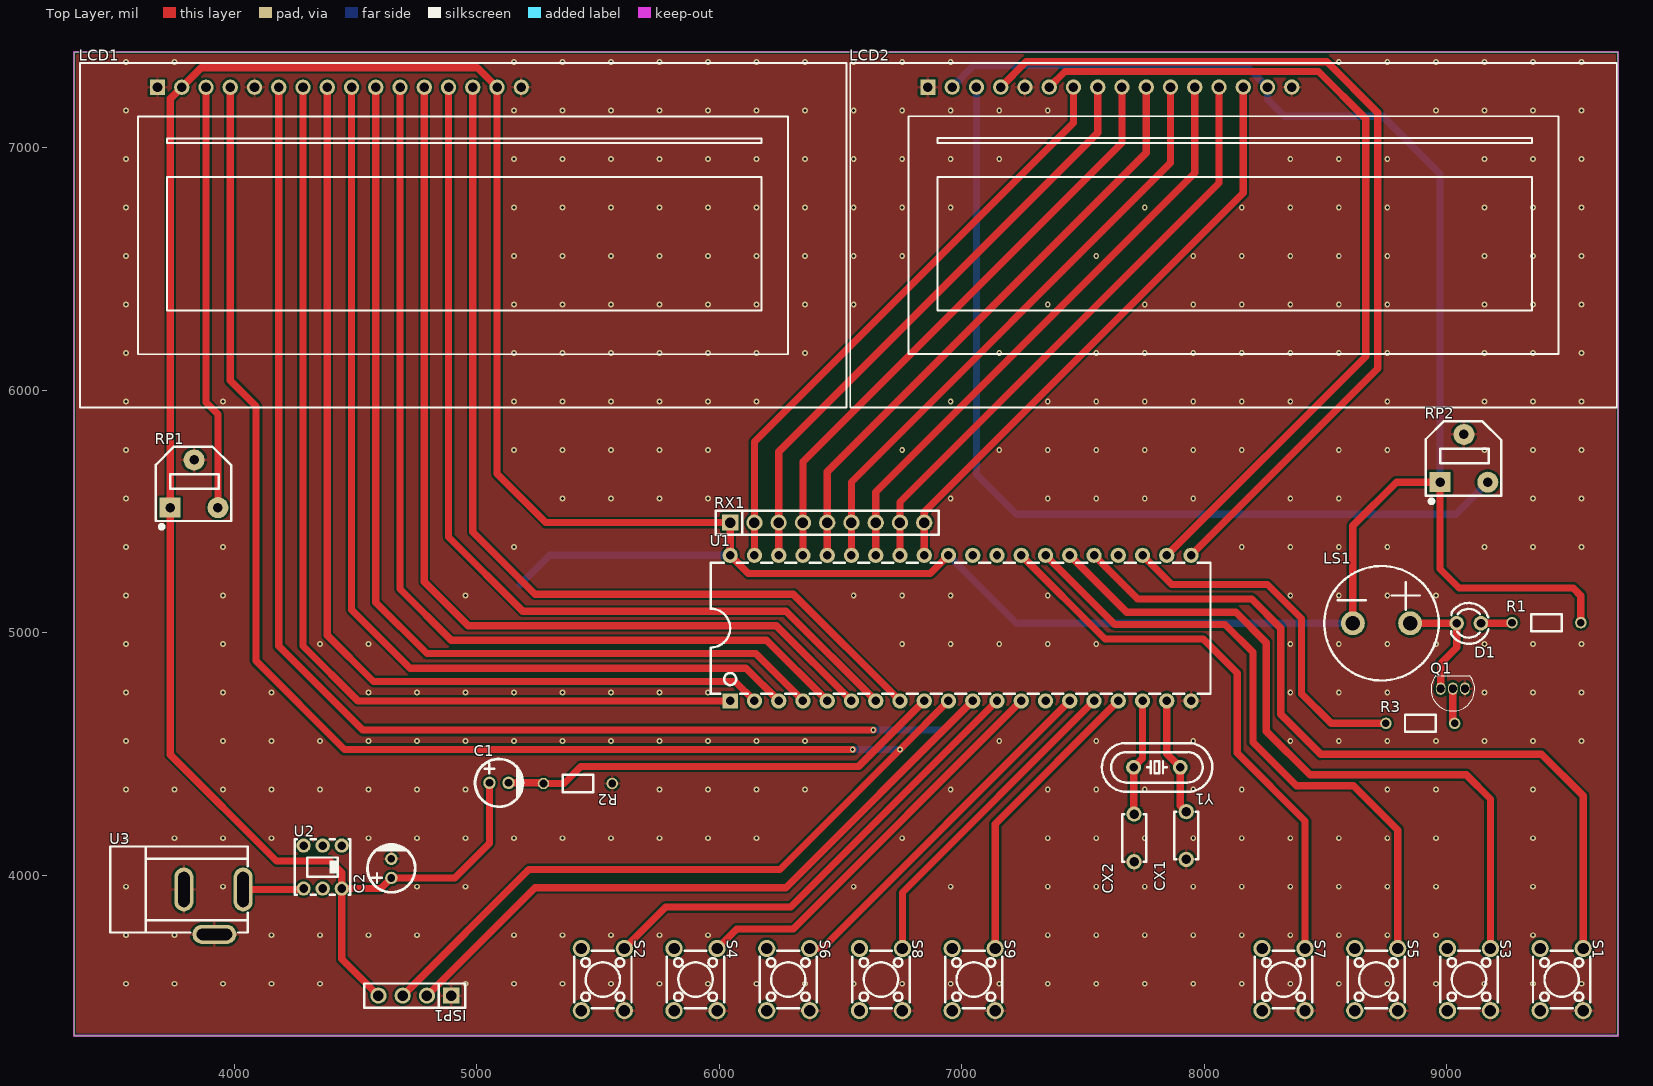
[diagram p0: Top Layer view]
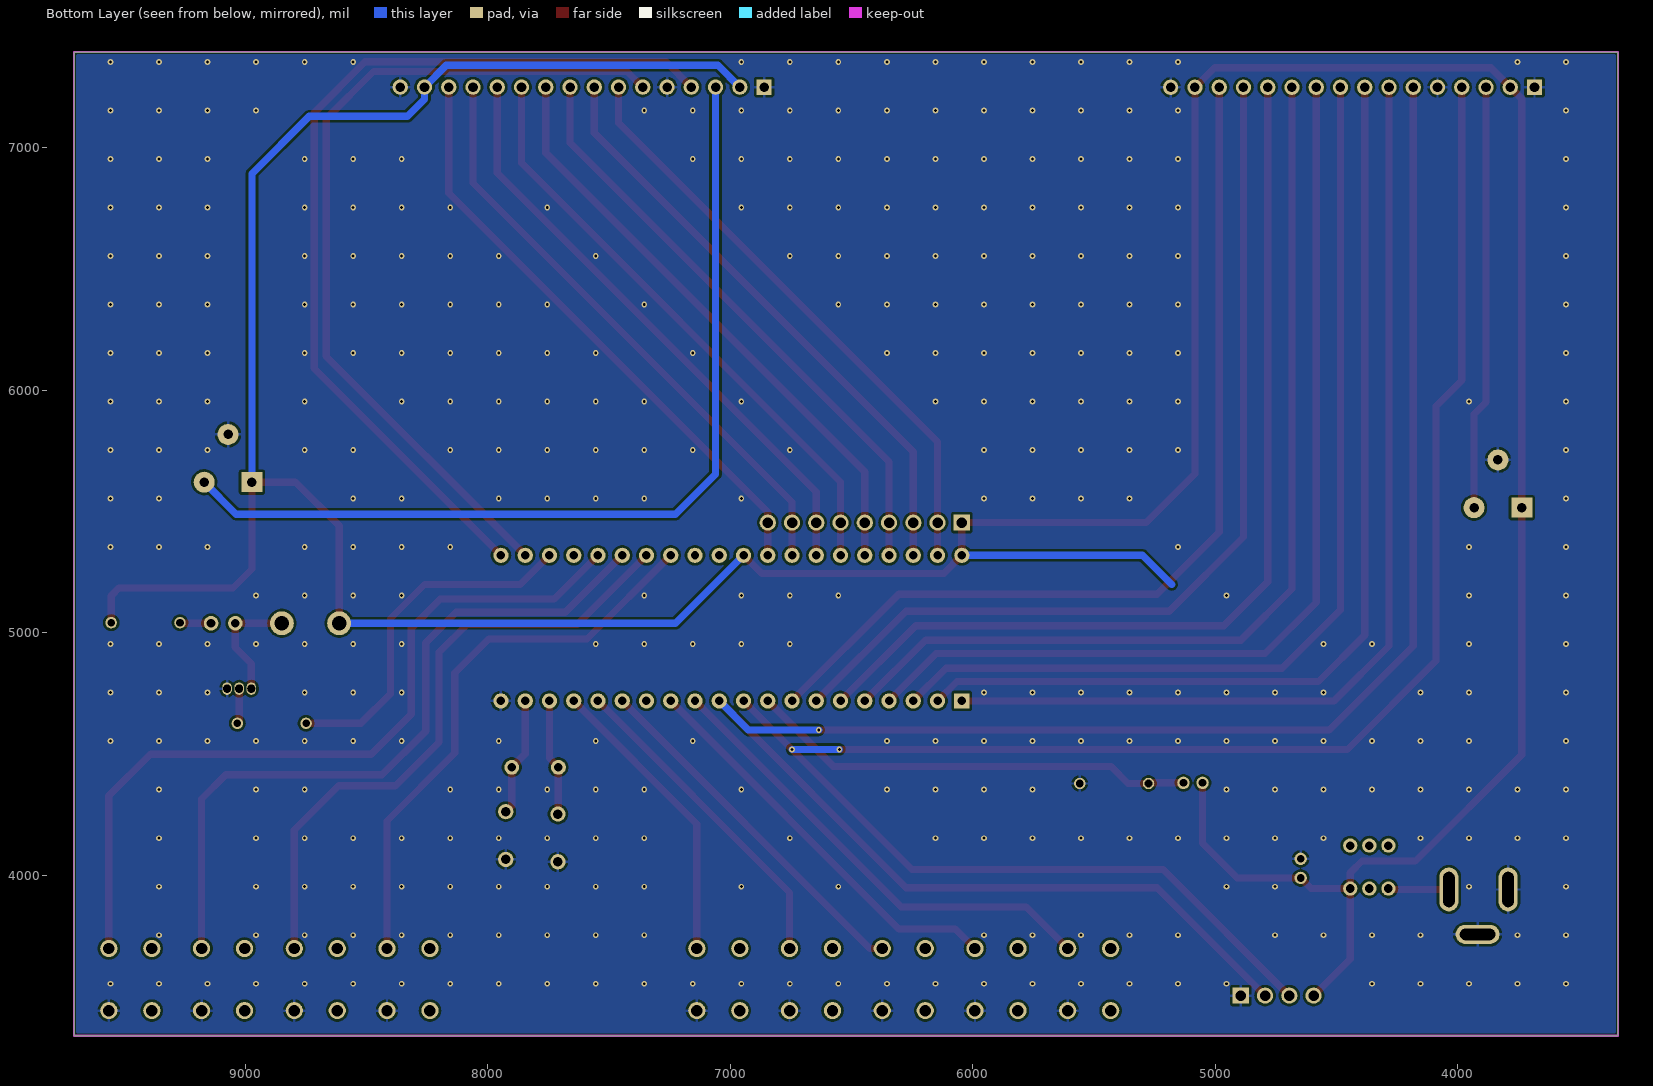
[diagram p1: Bottom Layer view, seen from below]
# Altium PCB MISC61252.pcbdoc
Units mil, origin at the board's own origin, x right, y up, seen from the top; angles counter-clockwise.
Board outline 6365 x 4055 mil, 2 copper layers (Top Layer, Bottom Layer), stack 62.206 mil thick; 29 components, 41 nets, 159 pads, 372 vias.

## Layer stack, top to bottom
Top Solder Mask Layer: solder mask 0.394, Dk 3.3
Top Layer: signal copper 1.379
Dielectric1: surface 59.449, FR4, Dk 4.5
Bottom Layer: signal copper 1.378
Bottom Solder Mask Layer: solder mask 0.394, Dk 3.3

## Board outline
3340,7395 3340,3340 9705,3340 9705,7395

## Design rules (kind name [scope] priority, off if disabled: settings)
BoardOutlineClearance copperThickness2oz_1 [All] p2 off: genericclearance=7.99 ignorepadtopadclearanceinfootprint=FALSE except(0: Arc-SplitContinuation Track-SplitContinuation SMDPad-SplitContinuation THPad-SplitContinuation Via-SplitContinuation Fill-SplitContinuation Region-SplitContinuation Poly-SplitContinuation Text-SplitContinuation Hole-SplitContinuation; 5.98: Arc-CutoutEdge SMDPad-CutoutEdge THPad-CutoutEdge Via-CutoutEdge Fill-CutoutEdge Region-CutoutEdge Text-CutoutEdge; 6.93: Hole-OutlineEdge Hole-CutoutEdge; 10: Poly-OutlineEdge Poly-CutoutEdge; 11.81: Arc-OutlineEdge Track-OutlineEdge SMDPad-OutlineEdge THPad-OutlineEdge Via-OutlineEdge Fill-OutlineEdge Region-OutlineEdge Text-OutlineEdge Track-CutoutEdge)
BoardOutlineClearance copperThickness1oz_1 [All] p4: genericclearance=4.02 ignorepadtopadclearanceinfootprint=FALSE except(0: Arc-SplitContinuation Track-SplitContinuation SMDPad-SplitContinuation THPad-SplitContinuation Via-SplitContinuation Fill-SplitContinuation Region-SplitContinuation Poly-SplitContinuation Text-SplitContinuation Hole-SplitContinuation; 6: SMDPad-CutoutEdge THPad-CutoutEdge Via-CutoutEdge Fill-CutoutEdge Region-CutoutEdge Text-CutoutEdge; 6.93: Hole-OutlineEdge Hole-CutoutEdge; 10: Poly-OutlineEdge Poly-CutoutEdge; 11.8: Arc-OutlineEdge Track-OutlineEdge SMDPad-OutlineEdge THPad-OutlineEdge Via-OutlineEdge Fill-OutlineEdge Region-OutlineEdge Text-OutlineEdge; 11.81: Arc-CutoutEdge Track-CutoutEdge)
Clearance copperThickness2oz [All] p1 off: gap=7.99 ignorepadtopadclearanceinfootprint=FALSE except(5.98: SMDPad-Track SMDPad-SMDPad THPad-Track SMDPad-THPad THPad-THPad Track-Via SMDPad-Via THPad-Via Via-Via Fill-Track Region-Track Fill-SMDPad Region-SMDPad Fill-THPad Region-THPad Fill-Via Region-Via Fill-Fill Fill-Region Region-Region Arc-Track Arc-SMDPad Arc-THPad Arc-Via Fill-Arc Region-Arc Arc-Arc Text-Track SMDPad-Text Text-THPad Text-Via Fill-Text Region-Text Arc-Text Text-Text; 6.93: Hole-Track Hole-SMDPad Hole-THPad Hole-Via Fill-Hole Region-Hole Hole-Arc Hole-Text; 10: Poly-Track Poly-SMDPad Poly-THPad Poly-Via Poly-Fill Poly-Region Poly-Poly Poly-Arc Poly-Text Poly-Hole)
Clearance copperThickness1oz [All] p3: gap=4.02 ignorepadtopadclearanceinfootprint=FALSE except(5.98: SMDPad-Track SMDPad-SMDPad THPad-Track SMDPad-THPad THPad-THPad Track-Via SMDPad-Via THPad-Via Via-Via Fill-Track Region-Track Fill-SMDPad Region-SMDPad Fill-THPad Region-THPad Fill-Via Region-Via Fill-Fill Fill-Region Region-Region; 6: Arc-Track Arc-SMDPad Arc-THPad Arc-Via Fill-Arc Region-Arc Arc-Arc Text-Track SMDPad-Text Text-THPad Text-Via Fill-Text Region-Text Arc-Text Text-Text; 6.93: Hole-Track Hole-SMDPad Hole-THPad Hole-Via Fill-Hole Region-Hole Hole-Arc Hole-Text; 10: Poly-Track Poly-SMDPad Poly-THPad Poly-Via Poly-Fill Poly-Region Poly-Poly Poly-Arc Poly-Text Poly-Hole)
Creepage creepage [All] p1: checkdistance=0 ignoreinternallayers=TRUE applytopolygonpour=TRUE
DiffPairsRouting differentialPair [All] p1: maxlimit=6 minlimit=6 mostfreqgap=6 toplayer_minwidth=5 toplayer_prefwidth=10 toplayer_maxwidth=100 toplayer_mingap=6 toplayer_prefgap=6 toplayer_maxgap=6 bottomlayer_minwidth=5 bottomlayer_prefwidth=10 bottomlayer_maxwidth=100 bottomlayer_mingap=6 bottomlayer_prefgap=6 bottomlayer_maxgap=6 maxuncoupledlength=10
HoleToHoleClearance otherClearance [All] p1: gap=11.81 allowstackedmicrovias=TRUE
Length netLength [All] p1: minlimit=0 maxlimit=0
MatchedLengths netLengthTolerance [All] p1: tolerance=1000
PasteMaskExpansion pasteMaskExpansion [All] p1: expansion=0
PlaneConnect innerPlane [All] p1: planeconnectstyle=Relief reliefexpansion=20 reliefentries=4 reliefconductorwidth=10 reliefairgap=10
PolygonConnect copperRegion [(InNet('GND'))] p1: connectstyle=Relief reliefconductorwidth=10 reliefentries=4 polygonreliefangle="90 Angle" airgapwidth=10 via.connectstyle=Relief via.reliefconductorwidth=10 via.reliefentries=4 via.polygonreliefangle="90 Angle" via.airgapwidth=10
RoutingVias viaSize [All] p1: holewidth=12.01 width=24.02 viastyle="Through Hole" minholewidth=11.81 minwidth=19.68 maxholewidth=248.03 maxwidth=393.7
SolderMaskExpansion solderMaskExpansion [IsVia] p1: expansion=-1000 istentingtop=TRUE
SolderMaskExpansion solderMaskExpansion [All] p2: expansion=2 istentingtop=FALSE
Width copperThickness2oz_2 [All] p1 off: maxlimit=100 minlimit=8 preferedwidth=10
Width copperThickness1oz_2 [All] p2: maxlimit=100 minlimit=5 preferedwidth=10

## Components (designator, comment, footprint, x,y, rotation, side; value= is the part's Value field where it differs from the comment)
C1 "Cap Pol2" CAP-TH_BD5.0-P2.00-D0.8-FD-10UF50VC110GL 5092.02,4382.02 r0 top
C2 "1000UF" CAP-TH_BD5.0-P2.00-D0.8-FD-10UF50VC110GL 4648.15,4029.51 r90 top
CX1 "Cap" CAP-TH_L5.0-W2.5-P5.00-D1.0 7925,4165 r90 top
CX2 "Cap" CAP-TH_L5.0-W2.5-P5.00-D1.0 7710,4155 r90 top
D1 "LED1" LED_TH-3mm 9090,5040 r180 top
ISP1 "Header 4" HDR-TH_4P-P2.54-V-F 4745,3505 r180 top
LCD1 "1602" LCD1602 4943.94,6639.21 r0 top
LCD2 "1602" LCD1602 8120,6640 r0 top
LS1 "Bell" BUZ-TH_BD12.0-P6.00-D0.9-RD 8730,5040 r0 top
Q1 "2N3906" TO-92-3_L4.6-W3.6-P1.27-L_1 9024.1,4770.58 r0 top
R1 "Res2" Res_1/8W 9410,5040 r0 top
R2 "Res2" Res_1/8W 5417.02,4382.02 r180 top
R3 "Res2" Res_1/8W 8890,4625 r0 top
RP1 "RPot" RES-ADJ-SMD_RM065-V1 3835,5615 r0 top
RP2 "RPot" RES-ADJ-SMD_RM065-V1 9070,5720 r0 top
RX1 "Header 9" HDR-TH_9P-P2.54-V-F-1 6445,5455 r0 top
S1 "SW-PB" SW-TH_4P-L6.0-W6.0-P4.50-LS6.5 9472.85,3571.25 r270 top
S2 "SW-PB" SW-TH_4P-L6.0-W6.0-P4.50-LS6.5 5520,3571.25 r270 top
S3 "SW-PB" SW-TH_4P-L6.0-W6.0-P4.50-LS6.5 9090.62,3571.25 r270 top
S4 "SW-PB" SW-TH_4P-L6.0-W6.0-P4.50-LS6.5 5902.23,3571.25 r270 top
S5 "SW-PB" SW-TH_4P-L6.0-W6.0-P4.50-LS6.5 8708.39,3571.25 r270 top
S6 "SW-PB" SW-TH_4P-L6.0-W6.0-P4.50-LS6.5 6284.46,3571.25 r270 top
S7 "SW-PB" SW-TH_4P-L6.0-W6.0-P4.50-LS6.5 8326.15,3571.25 r270 top
S8 "SW-PB" SW-TH_4P-L6.0-W6.0-P4.50-LS6.5 6666.69,3571.25 r270 top
S9 "SW-PB" SW-TH_4P-L6.0-W6.0-P4.50-LS6.5 7048.92,3571.25 r270 top
U1 "STC89C52" DIP-40_L52.0-W13.7-P2.54-LS15.2-BL 6995,5020 r0 top
U2 "SWITCH" SW-TH_6P-L5.8-W5.8-P2.00-LS4.5-BL 4365,4035 r0 top
U3 "POW" DC-IN-TH_DC005 3915,3850 r0 top
Y1 "XTAL" HC-49S_L11.5-W5.0-P4.88 7804.33,4446.25 r180 top

## Footprints (in the part's own frame and the unit in brackets; to place one, negate y for a bottom-side part, rotate by r counter-clockwise, add the part's x,y. Pads: shape width x height; smd on the part's side, far side on the other; paste and mask are expansions set on the pad)
BUZ-TH_BD12.0-P6.00-D0.9-RD [mm]
  round 2.5 hole 1.5 paste+0 mask+0.05: 1(-3,0) 2(3,0)
  silkscreen extent -5.99,-5.99 5.99,5.99
CAP-TH_BD5.0-P2.00-D0.8-FD-10UF50VC110GL [mm]
  round 1.3 hole 0.8: 1(-1,0) 2(1,0)
  silkscreen extent -2.5,-2.5 2.5,2.5
CAP-TH_L5.0-W2.5-P5.00-D1.0 [mm]
  round 1.6 hole 1: 1(-2.5,0) 2(2.5,0)
  silkscreen extent -2.5,-1.27 2.5,1.25
DC-IN-TH_DC005 [mm]
  oval 2x4.6 hole 1.2 slot 3.7 at 90 deg: 1(3.1,2.35) 2(-3.1,2.35)
  oval 4.6x2 hole 1.2 slot 3.7 at 0 deg: 3(0.1,-2.35)
  silkscreen extent -10.8,-2.15 3.6,6.85
DIP-40_L52.0-W13.7-P2.54-LS15.2-BL [mil]
  rect 63x63 hole 35: 1(-950,-300)
  round 63 hole 35: 2(-850,-300) 3(-750,-300) 4(-650,-300) 5(-550,-300) 6(-450,-300) 7(-350,-300) 8(-250,-300) 9(-150,-300) 10(-50,-300) 11(50,-300) 12(150,-300) 13(250,-300) 14(350,-300) 15(450,-300) 16(550,-300) 17(650,-300) 18(750,-300) 19(850,-300) 20(950,-300) 21(950,300) 22(850,300) 23(750,300) 24(650,300) 25(550,300) 26(450,300) 27(350,300) 28(250,300) 29(150,300) 30(50,300) 31(-50,300) 32(-150,300) 33(-250,300) 34(-350,300) 35(-450,300) 36(-550,300) 37(-650,300) 38(-750,300) 39(-850,300) 40(-950,300)
  silkscreen extent -1030,-270 1030,270
HC-49S_L11.5-W5.0-P4.88 [mm]
  round 1.56 hole 0.9: 1(-2.44,0) 2(2.44,0)
  silkscreen extent -5.8,-2.54 5.77,2.54
HDR-TH_4P-P2.54-V-F [mm]
  rect 1.7x1.7 hole 1.1: 1(-3.81,0)
  round 1.7 hole 1.1: 2(-1.27,0) 3(1.27,0) 4(3.81,0)
  silkscreen extent -5.29,-1.27 5.29,1.27
HDR-TH_9P-P2.54-V-F-1 [mm]
  rect 1.7x1.7 hole 1.1: 1(-10.16,0)
  round 1.7 hole 1.1: 2(-7.62,0) 3(-5.08,0) 4(-2.54,0) 5(0,0) 6(2.54,0) 7(5.08,0) 8(7.62,0) 9(10.16,0)
  silkscreen extent -11.68,-1.25 11.68,1.25
LCD1602 [mm]
  rect 1.6x1.6 hole 1: 1(-32,15.5)
  round 1.6 hole 1: 2(-29.46,15.5) 3(-26.92,15.5) 4(-24.38,15.5) 5(-21.84,15.5) 6(-19.3,15.5) 7(-16.76,15.5) 8(-14.22,15.5) 9(-11.68,15.5) 10(-9.14,15.5) 11(-6.6,15.5) 12(-4.06,15.5) 13(-1.52,15.5) 14(1.02,15.5) 15(3.56,15.5) 16(6.1,15.5)
  silkscreen extent -40.13,-18.03 40.13,18.03
LED_TH-3mm [mil]
  round 60 hole 36 paste+0 mask+2: 1(-50,0) 2(50,0)
  silkscreen extent -81,-84 72,85
RES-ADJ-SMD_RM065-V1 [mm]
  rect 2.2x2.1 hole 1 paste+0 mask+0.05: 1(-2.5,-2.5)
  round 2.2 hole 1 paste+0 mask+0.05: 2(0,2.5) 3(2.5,-2.5)
  silkscreen extent -4,-4.7 3.9,3.9
Res_1/8W [mil]
  round 47.2 hole 31.5 paste+0 mask+2: 1(-141.7,2.48) 2(141.7,2.48)
  silkscreen extent -63,-33 63,38
SW-TH_4P-L6.0-W6.0-P4.50-LS6.5 [mm]
  round 1.8 hole 1.2: 1(-3.25,2.25) 2(3.25,2.25) 3(-3.25,-2.25) 4(3.25,-2.25)
  silkscreen extent -3,-3 3,3
SW-TH_6P-L5.8-W5.8-P2.00-LS4.5-BL [mm]
  round 1.5 hole 0.9 paste+0 mask+0.05: 1(-2,-2.25) 2(0,-2.25) 3(2,-2.25) 4(-2,2.25) 5(0,2.25) 6(2,2.25)
  silkscreen extent -2.9,-2.9 2.9,2.9
TO-92-3_L4.6-W3.6-P1.27-L_1 [mm]
  oval 1x1.3 hole 0.8 slot 0.84 at 90 deg paste+0 mask+0.05: 1(-1.27,0) 2(0,0) 3(1.27,0)
  silkscreen extent -2.28,-2.34 2.28,1.35

## Via types
v1: diameter 24.02, hole 12, Top Layer to Bottom Layer, 372 vias

## Nets (pads, with @x,y where several pads share a name; then routed paths per layer and width w, separated by ;. In a path a pad name is that pad's centre, name@x,y a point inside that pad or via, vN(x,y) a via of type N, cw(c..) or ccw(c..) an arc to the next point about the centre after c; other vN are vias at no path point)
$1N1: D1.1 R1.1 | length 129.3
  Top Layer w30: D1.1 9265.82,5040 R1.1
$1N2: Q1.2 R3.2 | length 146.3
  Top Layer w30: Q1.2 9024.1,4635.08 R3.2
$1N19: U2.1 U3.1 | length 250.8
  Top Layer w30: U3.1 4282.35,3942.51 U2.1
$1N20: S7.1 U1.28 | length 2342.6
  Top Layer w30: U1.28 7590,4975 7995,4975 8135,4835 8135,4505 8414.73,4225.27 S7.1
$1N21: S5.1 U1.27 | length 2626.4
  Top Layer w30: U1.27 7630,5035 8085,5035 8200,4920 8200,4550 8380,4370 8615,4370 8796.97,4188.03 S5.1
$1N22: S3.1 U1.26 | length 2980.6
  Top Layer w30: U1.26 7680,5085 8130,5085 8255,4960 8255,4595 8435,4415 9080,4415 9179.2,4315.8 S3.1
$1N23: S1.1 U1.25 | length 3264.4
  Top Layer w30: U1.25 7725,5140 8195,5140 8315,5020 8315,4665 8480,4500 9390,4500 9561.43,4328.57 S1.1
$1N24: S4.1 U1.13 | length 1677
  Top Layer w30: S4.1 6071.61,3780 6305,3780 U1.13
$1N25: S9.1 U1.17 | length 1231
  Top Layer w30: S9.1 7137.5,4212.5 U1.17
$1N26: S8.1 U1.16 | length 1347.9
  Top Layer w30: S8.1 6755.27,3930.27 U1.16
$1N27: S6.1 U1.15 | length 1494.8
  Top Layer w30: S6.1 6424.2,3699.2 U1.15
$1N28: S2.1 U1.12 | length 1959.3
  Top Layer w30: S2.1 5779.38,3870 6295,3870 U1.12
$1N29: CX1.2 U1.19 Y1.1 | length 489.7
  Top Layer w30: U1.19 7845,4501.63 Y1.1 7900.39,4288.04 CX1.2
$1N32: LCD1.7 U1.1 | length 4158
  Top Layer w30: LCD1.7 4284.1,4945.9 4510,4720 U1.1
$1N33: LCD1.8 U1.2 | length 4131.7
  Top Layer w30: LCD1.8 4384.1,4990.9 4575,4800 6065,4800 U1.2
$1N34: LCD1.9 U1.3 | length 4070.2
  Top Layer w30: LCD1.9 4484.1,5095.9 4725,4855 6110,4855 U1.3
$1N35: LCD1.10 U1.4 | length 4052.6
  Top Layer w30: LCD1.10 4584.1,5125.9 4795,4915 6150,4915 U1.4
$1N36: LCD1.11 U1.5 | length 4020.4
  Top Layer w30: LCD1.11 4684.1,5180.9 4895,4970 6195,4970 U1.5
$1N37: LCD1.12 U1.6 | length 4002.8
  Top Layer w30: LCD1.12 4784.1,5210.9 4965,5030 6235,5030 U1.6
$1N38: LCD1.13 U1.7 | length 3894.4
  Top Layer w30: LCD1.13 4884.1,5395.9 5190,5090 6275,5090 U1.7
$1N39: LCD1.14 U1.8 | length 3882.7
  Top Layer w30: LCD1.14 4984.1,5415.9 5240,5160 6305,5160 U1.8
$1N42: LCD1.3 RP1.3 | length 1753.3
  Top Layer w30: LCD1.3 3884.09,5950.9 3933.43,5901.57 RP1.3
$1N44: R3.1 U1.23 | length 1471.7
  Top Layer w30: U1.23 7865,5200 8260,5200 8400,5060 8400,4750 8522.52,4627.48 R3.1
$1N45: LCD2.6 U1.22 | length 3552.1
  Top Layer w30: LCD2.6 7424.92,7315 8470,7315 8665,7120 8665,6140 U1.22
$1N46: LCD2.4 U1.21 | length 3829.2
  Top Layer w30: LCD2.4 7264.92,7355 8505,7355 8715,7145 8715,6090 U1.21
$1N48: D1.2 LS1.2 Q1.1 | length 488.6
  Top Layer w30: LS1.2 D1.2 9040,4940 8974.1,4874.1 Q1.1
$1N51: CX2.2 U1.18 Y1.2 | length 482.5
  Top Layer w30: CX2.2 7708.27,4255.16 Y1.2 7745,4482.98 U1.18
$1N53: LCD2.3 RP2.3 | length 3826.4
  Bottom Layer w30: LCD2.3 7060.16,5654.84 7225,5490 9036.85,5490 RP2.3
$1N56: LCD2.14 RX1.9 U1.32 | length 2475
  Top Layer w30: U1.32 RX1.9 6845,5498.46 8160.16,6813.62 LCD2.14
$1N57: LCD2.13 RX1.8 U1.33 | length 2475
  Top Layer w30: U1.33 RX1.8 6745,5539.89 8060.16,6855.05 LCD2.13
$1N58: LCD2.12 RX1.7 U1.34 | length 2475
  Top Layer w30: U1.34 RX1.7 6645,5581.31 7960.16,6896.47 LCD2.12
$1N59: LCD2.11 RX1.6 U1.35 | length 2475
  Top Layer w30: U1.35 RX1.6 6545,5622.73 7860.16,6937.89 LCD2.11
$1N60: LCD2.10 RX1.5 U1.36 | length 2475
  Top Layer w30: U1.36 RX1.5 6445,5664.15 7760.16,6979.31 LCD2.10
$1N61: LCD2.9 RX1.4 U1.37 | length 2475
  Top Layer w30: U1.37 RX1.4 6345,5705.57 7660.16,7020.73 LCD2.9
$1N62: LCD2.8 RX1.3 U1.38 | length 2475
  Top Layer w30: U1.38 RX1.3 6245,5746.99 7560.16,7062.15 LCD2.8
$1N63: LCD2.7 RX1.2 U1.39 | length 2475
  Top Layer w30: U1.39 RX1.2 6145,5788.41 7460.16,7103.57 LCD2.7
GND: C2.2 CX1.1 CX2.1 ISP1.1 LCD1.1 LCD1.5 LCD1.16 LCD2.1 LCD2.5 LCD2.16 Q1.3 R2.1 RP1.2 RP2.2 S1.2 S2.2 S3.2 S4.2 S5.2 S6.2 S7.2 S8.2 S9.2 U1.20 U3.2 U3.3
  other v1: 3554.1,3554.1 3754.1,3554.1 3954.1,3554.1 4154.1,3554.1 4354.1,3554.1 4954.1,3554.1 5154.1,3554.1 5354.1,3554.1 5554.1,3554.1 5754.1,3554.1 5954.1,3554.1 6154.1,3554.1 6354.1,3554.1 6554.1,3554.1 6754.1,3554.1 6954.1,3554.1 7154.1,3554.1 7354.1,3554.1 7554.1,3554.1 7754.1,3554.1 7954.1,3554.1 8154.1,3554.1 8354.1,3554.1 8554.1,3554.1 8754.1,3554.1 8954.1,3554.1 9154.1,3554.1 9354.1,3554.1 9554.1,3554.1 3554.1,3754.1 3754.1,3754.1 4154.1,3754.1 4354.1,3754.1 4554.1,3754.1 4754.1,3754.1 5154.1,3754.1 5354.1,3754.1 5554.1,3754.1 5754.1,3754.1 5954.1,3754.1 7354.1,3754.1 7554.1,3754.1 7754.1,3754.1 7954.1,3754.1 8154.1,3754.1 8354.1,3754.1 8554.1,3754.1 8754.1,3754.1 8954.1,3754.1 9354.1,3754.1 3554.1,3954.1 3954.1,3954.1 4754.1,3954.1 4954.1,3954.1 6554.1,3954.1 6954.1,3954.1 7354.1,3954.1 7554.1,3954.1 7754.1,3954.1 7954.1,3954.1 8154.1,3954.1 8354.1,3954.1 8554.1,3954.1 8754.1,3954.1 8954.1,3954.1 9354.1,3954.1 3554.1,4154.1 3754.1,4154.1 3954.1,4154.1 4154.1,4154.1 4554.1,4154.1 4754.1,4154.1 4954.1,4154.1 5154.1,4154.1 5354.1,4154.1 5554.1,4154.1 5754.1,4154.1 5954.1,4154.1 6154.1,4154.1 6754.1,4154.1 7354.1,4154.1 7554.1,4154.1 7754.1,4154.1 7954.1,4154.1 8154.1,4154.1 8354.1,4154.1 8554.1,4154.1 8754.1,4154.1 8954.1,4154.1 9354.1,4154.1 3554.1,4354.1 3754.1,4354.1 3954.1,4354.1 4154.1,4354.1 4354.1,4354.1 4554.1,4354.1 4754.1,4354.1 4954.1,4354.1 5754.1,4354.1 5954.1,4354.1 6154.1,4354.1 6354.1,4354.1 6954.1,4354.1 7354.1,4354.1 7554.1,4354.1 7754.1,4354.1 7954.1,4354.1 8154.1,4354.1 8754.1,4354.1 8954.1,4354.1 9354.1,4354.1 3554.1,4554.1 3954.1,4554.1 4154.1,4554.1 4354.1,4554.1 4554.1,4554.1 4754.1,4554.1 4954.1,4554.1 5154.1,4554.1 5354.1,4554.1 5554.1,4554.1 5754.1,4554.1 5954.1,4554.1 6154.1,4554.1 6354.1,4554.1 7154.1,4554.1 7554.1,4554.1 7954.1,4554.1 8354.1,4554.1 8554.1,4554.1 8754.1,4554.1 8954.1,4554.1 9154.1,4554.1 9354.1,4554.1 9554.1,4554.1 3554.1,4754.1 3954.1,4754.1 4154.1,4754.1 4554.1,4754.1 4754.1,4754.1 4954.1,4754.1 5154.1,4754.1 5354.1,4754.1 5554.1,4754.1 5754.1,4754.1 5954.1,4754.1 8354.1,4754.1 8554.1,4754.1 8754.1,4754.1 9154.1,4754.1 9354.1,4754.1 9554.1,4754.1 3554.1,4954.1 3954.1,4954.1 4354.1,4954.1 4554.1,4954.1 6754.1,4954.1 6954.1,4954.1 7154.1,4954.1 7354.1,4954.1 7554.1,4954.1 8354.1,4954.1 8554.1,4954.1 8754.1,4954.1 8954.1,4954.1 9154.1,4954.1 9354.1,4954.1 9554.1,4954.1 3554.1,5154.1 3954.1,5154.1 4954.1,5154.1 6554.1,5154.1 6754.1,5154.1 6954.1,5154.1 7354.1,5154.1 8354.1,5154.1 8554.1,5154.1 8754.1,5154.1 8954.1,5154.1 3554.1,5354.1 3954.1,5354.1 5154.1,5354.1 8154.1,5354.1 8354.1,5354.1 8554.1,5354.1 8754.1,5354.1 9154.1,5354.1 9354.1,5354.1 9554.1,5354.1 3554.1,5554.1 5354.1,5554.1 5554.1,5554.1 5754.1,5554.1 5954.1,5554.1 6954.1,5554.1 7354.1,5554.1 7554.1,5554.1 7754.1,5554.1 7954.1,5554.1 8354.1,5554.1 8554.1,5554.1 9354.1,5554.1 9554.1,5554.1 3554.1,5754.1 5154.1,5754.1 5354.1,5754.1 5554.1,5754.1 5754.1,5754.1 5954.1,5754.1 6754.1,5754.1 7154.1,5754.1 7354.1,5754.1 7554.1,5754.1 7754.1,5754.1 7954.1,5754.1 8154.1,5754.1 8554.1,5754.1 8754.1,5754.1 9154.1,5754.1 9354.1,5754.1 9554.1,5754.1 3554.1,5954.1 3954.1,5954.1 5154.1,5954.1 5354.1,5954.1 5554.1,5954.1 5754.1,5954.1 5954.1,5954.1 6154.1,5954.1 6954.1,5954.1 7354.1,5954.1 7554.1,5954.1 7754.1,5954.1 7954.1,5954.1 8154.1,5954.1 8354.1,5954.1 8754.1,5954.1 9154.1,5954.1 9354.1,5954.1 9554.1,5954.1 3554.1,6154.1 5154.1,6154.1 5354.1,6154.1 5554.1,6154.1 5754.1,6154.1 5954.1,6154.1 6154.1,6154.1 6354.1,6154.1 7154.1,6154.1 7554.1,6154.1 7754.1,6154.1 7954.1,6154.1 8154.1,6154.1 8354.1,6154.1 8554.1,6154.1 8754.1,6154.1 9154.1,6154.1 9354.1,6154.1 9554.1,6154.1 3554.1,6354.1 5154.1,6354.1 5354.1,6354.1 5554.1,6354.1 5754.1,6354.1 5954.1,6354.1 6154.1,6354.1 6354.1,6354.1 6554.1,6354.1 7354.1,6354.1 7754.1,6354.1 7954.1,6354.1 8154.1,6354.1 8354.1,6354.1 8554.1,6354.1 8754.1,6354.1 9154.1,6354.1 9354.1,6354.1 9554.1,6354.1 3554.1,6554.1 5154.1,6554.1 5354.1,6554.1 5554.1,6554.1 5754.1,6554.1 5954.1,6554.1 6154.1,6554.1 6354.1,6554.1 6554.1,6554.1 6754.1,6554.1 7554.1,6554.1 7954.1,6554.1 8154.1,6554.1 8354.1,6554.1 8554.1,6554.1 8754.1,6554.1 9154.1,6554.1 9354.1,6554.1 9554.1,6554.1 3554.1,6754.1 5154.1,6754.1 5354.1,6754.1 5554.1,6754.1 5754.1,6754.1 5954.1,6754.1 6154.1,6754.1 6354.1,6754.1 6554.1,6754.1 6754.1,6754.1 6954.1,6754.1 7754.1,6754.1 8154.1,6754.1 8354.1,6754.1 8554.1,6754.1 8754.1,6754.1 9154.1,6754.1 9354.1,6754.1 9554.1,6754.1 3554.1,6954.1 5154.1,6954.1 5354.1,6954.1 5554.1,6954.1 5754.1,6954.1 5954.1,6954.1 6154.1,6954.1 6354.1,6954.1 6554.1,6954.1 6754.1,6954.1 6954.1,6954.1 7154.1,6954.1 8354.1,6954.1 8554.1,6954.1 8754.1,6954.1 9154.1,6954.1 9354.1,6954.1 9554.1,6954.1 3554.1,7154.1 5154.1,7154.1 5354.1,7154.1 5554.1,7154.1 5754.1,7154.1 5954.1,7154.1 6154.1,7154.1 6354.1,7154.1 6554.1,7154.1 6754.1,7154.1 6954.1,7154.1 7154.1,7154.1 7354.1,7154.1 8954.1,7154.1 9154.1,7154.1 9354.1,7154.1 9554.1,7154.1 3554.1,7354.1 3754.1,7354.1 5154.1,7354.1 5354.1,7354.1 5554.1,7354.1 5754.1,7354.1 5954.1,7354.1 6154.1,7354.1 6354.1,7354.1 6554.1,7354.1 6754.1,7354.1 6954.1,7354.1 8554.1,7354.1 8754.1,7354.1 8954.1,7354.1 9154.1,7354.1 9354.1,7354.1 9554.1,7354.1
RST: C1.2 R2.2 U1.9 | length 1855.7
  Top Layer w30: C1.2 5272.84,4382.02 R2.2 5359.54,4379.54 5430,4450 6575,4450 U1.9
RXD: ISP1.3 LCD1.4 U1.10 | length 7967.8
  Top Layer w30: LCD1.4 3984.09,6040.9 4090,5935 4090,4885 4455,4520 v1(6550,4520) ; ISP1.3 5215,4025 6250,4025 v1(6745,4520) U1.10
  Bottom Layer w30: v1(6550,4520) v1(6745,4520)
TXD: ISP1.2 LCD1.6 U1.11 | length 8110.7
  Top Layer w30: LCD1.6 4184.1,4945.9 4530,4600 v1(6635,4600) ; ISP1.2 5240,3950 6275,3950 U1.11
  Bottom Layer w30: v1(6635,4600) 6925,4600 U1.11
VCC: C1.1 C2.1 ISP1.4 LCD1.2 LCD1.15 LCD2.2 LCD2.15 LS1.1 R1.2 RP1.1 RP2.1 RX1.1 U1.31 U1.40 U2.3 | length 18448.8
  Top Layer w30: ISP1.4 4443.74,3656.26 U2.3 ; C1.1 5052.65,4132.65 4910.14,3990.14 C2.1 4604.43,3946.42 U2.3 ; U1.31 6870,5245 6120,5245 U1.40 RX1.1 5285,5455 5084.1,5655.9 LCD1.15 5003.55,7330 3864.64,7330 LCD1.2 3736.57,7201.93 RP1.1 3736.57,4498.43 4175,4060 4395,4060 4443.74,4011.26 U2.3 ; LS1.1 8611.89,5441.89 8791.58,5621.57 RP2.1 8971.58,5263.43 9050,5185 9520,5185 9551.7,5153.3 R1.2
  Bottom Layer w30: 5180,5200 5300,5320 U1.40 ; U1.31 7225,5040 LS1.1 ; LCD2.2 7049.92,7340 8170.4,7340 LCD2.15 8260.16,7199.84 8330,7130 8735,7130 8971.58,6893.43 RP2.1
pads on no net: S1.3 S1.4 S2.3 S2.4 S3.3 S3.4 S4.3 S4.4 S5.3 S5.4 S6.3 S6.4 S7.3 S7.4 S8.3 S8.4 S9.3 S9.4 U1.14 U1.24 U1.29 U1.30 U2.2 U2.4 U2.5 U2.6

## Polygon pours and split planes (outlines as drawn)
GND on Top Layer (solid, remove dead copper, pour order 0): 3145,8135 3145,3000 10210,3000 10210,8135
GND on Bottom Layer (solid, remove dead copper, pour order 2): 3000,7845 3000,3215 10325,3215 10325,7845

## Keep-outs
Board Outline Layer:
  the board outline again, w10